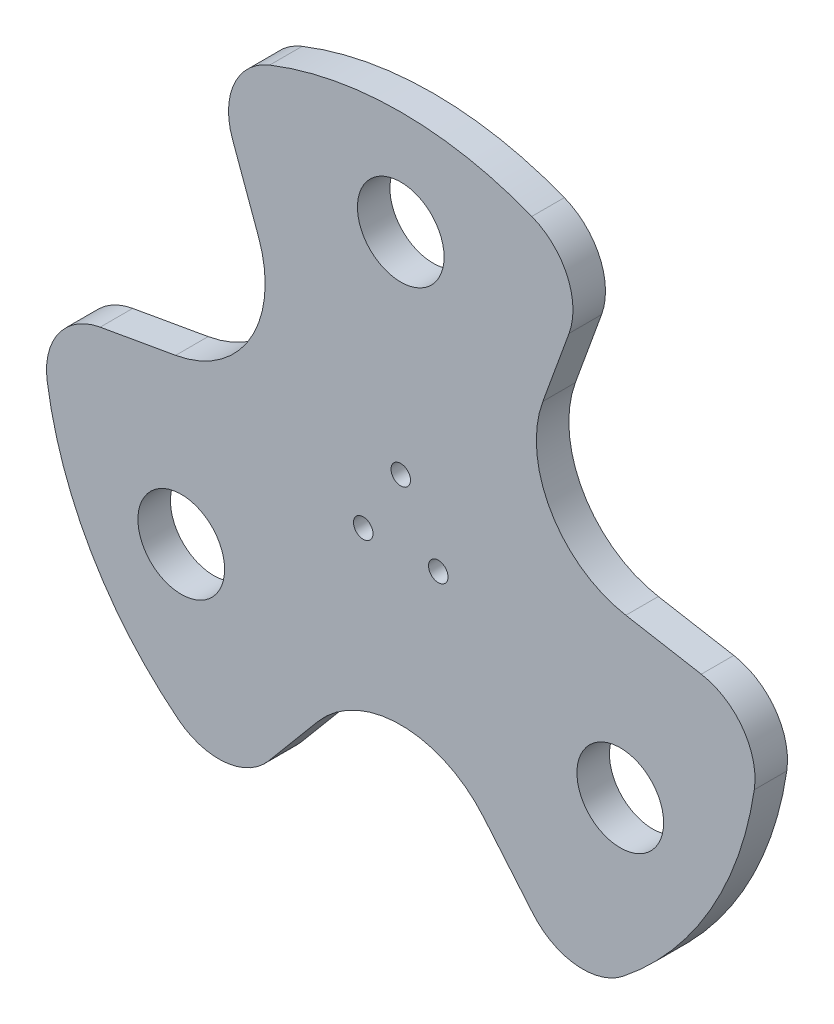
from build123d import *

# Parameters (mm, degrees)
SKETCH1_R           = 165
SKETCH1_R_2         = 20
BOSS_EXTRUDE1_DEPTH = 15
CUT_EXTRUDE1_DEPTH  = 30
FILLET1_R           = 30
SKETCH3_R           = 4.5
CUT_EXTRUDE2_DEPTH  = 20


with BuildPart() as part:
    # Sketch1 → Boss-Extrude1 (new body)
    with BuildSketch(Plane.XY):
        Circle(SKETCH1_R)
        with Locations((0, 117)):
            Circle(SKETCH1_R_2, mode=Mode.SUBTRACT)
        with Locations((101.324972243, -58.5)):
            Circle(SKETCH1_R_2, mode=Mode.SUBTRACT)
        with Locations((-101.324972243, -58.5)):
            Circle(SKETCH1_R_2, mode=Mode.SUBTRACT)
    extrude(amount=BOSS_EXTRUDE1_DEPTH)

    # Sketch2 → Cut-Extrude1 (cut)
    with BuildSketch(Plane.XY.offset(15)):
        with BuildLine():
            Line((-38.302222156, -97.860619516), (-169.990854036, -254.801019663))
            Line((-169.990854036, -254.801019663), (115.890035572, -190.326174896))
            Line((115.890035572, -190.326174896), (38.302222156, -97.860619516))
            ThreePointArc((38.302222156, -97.860619516), (0, -80), (-38.302222156, -97.860619516))
        make_face()
        with BuildLine():
            Line((-65.598671453, 82.101007166), (-135.66872892, 274.616907838))
            Line((-135.66872892, 274.616907838), (-222.772320251, -5.200627403))
            Line((-222.772320251, -5.200627403), (-103.900893609, 15.759612349))
            ThreePointArc((-103.900893609, 15.759612349), (-69.282032303, 40), (-65.598671453, 82.101007166))
        make_face()
        with BuildLine():
            Line((103.900893609, 15.759612349), (305.659582957, -19.815888175))
            Line((305.659582957, -19.815888175), (106.882284679, 195.526802298))
            Line((106.882284679, 195.526802298), (65.598671453, 82.101007166))
            ThreePointArc((65.598671453, 82.101007166), (69.282032303, 40), (103.900893609, 15.759612349))
        make_face()
    extrude(amount=-CUT_EXTRUDE1_DEPTH, mode=Mode.SUBTRACT)

    # Fillet1
    fillet1_edges = [part.edges().sort_by_distance(p)[0] for p in [
        (164.924238662, 4.999550163, 7.5),
        (86.79185678, 140.328805299, 7.5),
        (-86.79185678, 140.328805299, 7.5),
        (-164.924238662, 4.999550163, 7.5),
        (-78.132381882, -145.328355463, 7.5),
        (78.132381882, -145.328355463, 7.5),
    ]]
    fillet(fillet1_edges, radius=FILLET1_R)

    # Sketch3 → Cut-Extrude2 (cut)
    with BuildSketch(Plane.XY.offset(15)):
        with Locations((0, 20)):
            Circle(SKETCH3_R)
        with Locations((17.320508076, -10)):
            Circle(SKETCH3_R)
        with Locations((-17.320508076, -10)):
            Circle(SKETCH3_R)
    extrude(amount=-CUT_EXTRUDE2_DEPTH, mode=Mode.SUBTRACT)


solid = part.part
